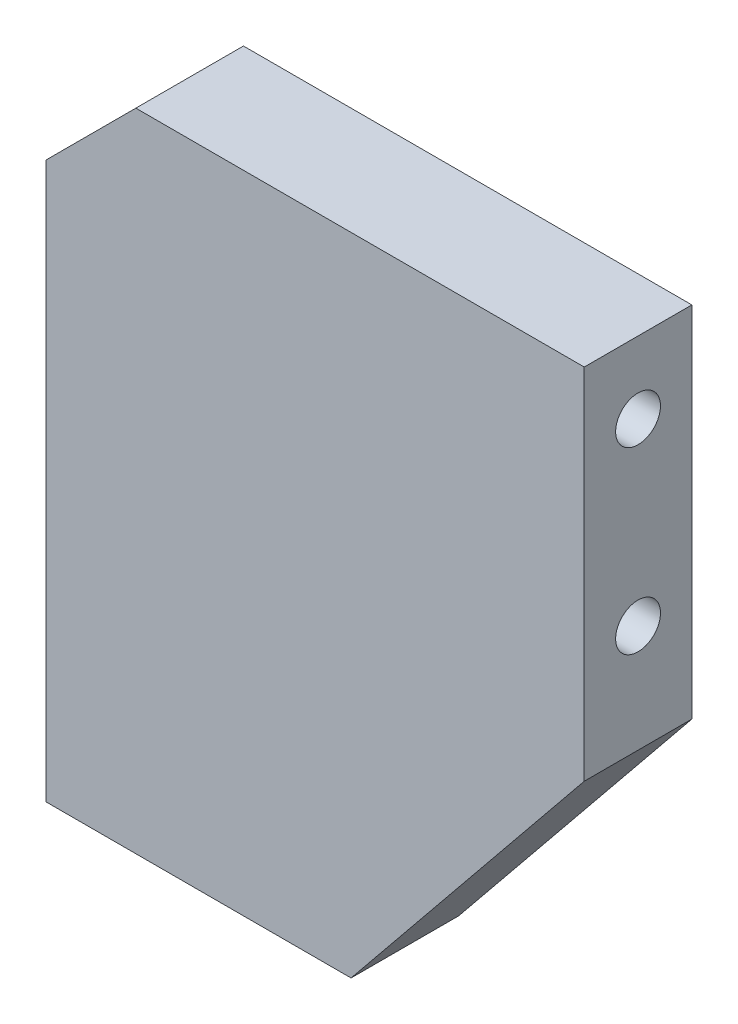
from build123d import *

# Parameters (mm, degrees)
EXTRUDE_1_DEPTH        = 12
CHAMFER_1_SIZE         = 10
HOLE_WIZARD_M6_1_D     = 5
HOLE_WIZARD_M6_1_DEPTH = 13
HOLE_WIZARD_M6_1_TIP   = 1.502151548
HOLE_WIZARD_M6_2_D     = 5
HOLE_WIZARD_M6_2_DEPTH = 13
HOLE_WIZARD_M6_2_TIP   = 1.502151548


with BuildPart() as part:
    # 草图1 → 凸台-拉伸1 (new body)
    with BuildSketch(Plane.XY):
        Polygon((-39.998611317, 12), (-39.998611317, -28), (-65.998611317, -60), (-99.998611317, -60), (-99.998611317, 12), align=None)
    extrude(amount=EXTRUDE_1_DEPTH)

    # 倒角1
    chamfer_1_edges = [part.edges().sort_by_distance(p)[0] for p in [
        (-99.998611317, 12, 6),
    ]]
    chamfer(chamfer_1_edges, length=CHAMFER_1_SIZE)

    # M6 螺纹孔1
    with Locations(Plane(origin=(-39.998611317, 0, 0), x_dir=(0, 0, -1), z_dir=(1, 0, 0))):
        with Locations((-6, 4), (-6, -16)):
            Hole(HOLE_WIZARD_M6_1_D / 2, depth=HOLE_WIZARD_M6_1_DEPTH)
            with Locations((0, 0, -(HOLE_WIZARD_M6_1_DEPTH + HOLE_WIZARD_M6_1_TIP / 2))):  # 118° drill point
                Cone(0, HOLE_WIZARD_M6_1_D / 2, HOLE_WIZARD_M6_1_TIP, mode=Mode.SUBTRACT)

    # M6 螺纹孔2
    with Locations(Plane.ZY.offset(99.998611317)):
        with Locations((6, -8), (6, -48)):
            Hole(HOLE_WIZARD_M6_2_D / 2, depth=HOLE_WIZARD_M6_2_DEPTH)
            with Locations((0, 0, -(HOLE_WIZARD_M6_2_DEPTH + HOLE_WIZARD_M6_2_TIP / 2))):  # 118° drill point
                Cone(0, HOLE_WIZARD_M6_2_D / 2, HOLE_WIZARD_M6_2_TIP, mode=Mode.SUBTRACT)


solid = part.part
